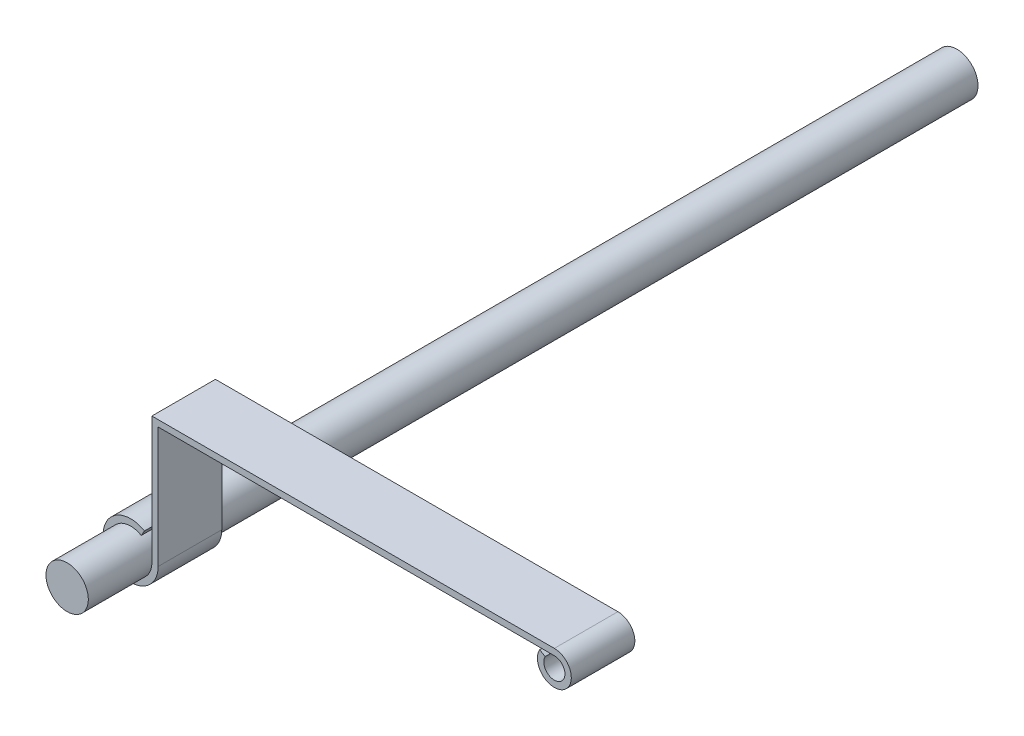
from build123d import *

# Parameters (mm, degrees)
SKETCH1_W           = 10
SKETCH1_H           = 30
BOSS_EXTRUDE1_START = 30
BOSS_EXTRUDE1_DEPTH = 30
BOSS_EXTRUDE2_START = 360
SKETCH3_R           = 10
BOSS_EXTRUDE2_DEPTH = 360


with BuildPart() as part:
    # Sketch1 → Revolve1 (revolve)
    with BuildSketch(Plane(origin=(0, 0, 0), x_dir=(1, 0, 0), z_dir=(0, 1, 0))):
        with Locations((5, -30)):
            Rectangle(SKETCH1_W, SKETCH1_H)
    revolve(axis=Axis((0, 0, 15), (0, 0, 1)))

    # Sketch2 → Boss-Extrude1 (add)
    with BuildSketch(Plane(origin=(0, 0, 15), x_dir=(-1, 0, 0), z_dir=(0, 0, -1)).offset(BOSS_EXTRUDE1_START)):
        with BuildLine():
            Line((-5, 8.660254038), (-6.5, 11.258330249))
            ThreePointArc((-6.5, 11.258330249), (11.258330249, -6.5), (-13, 0))
            Line((-13, 0), (-13, 57))
            Line((-13, 57), (-200, 57))
            ThreePointArc((-200, 57), (-202.5, 47.669872981), (-195.669872981, 54.5))
            Line((-195.669872981, 54.5), (-193.07179677, 56))
            ThreePointArc((-193.07179677, 56), (-204, 45.07179677), (-200, 60))
            Line((-200, 60), (-10, 60))
            Line((-10, 60), (-10, 0))
            ThreePointArc((-10, 0), (-8.660254038, 5), (-5, 8.660254038))
        make_face()
    extrude(amount=-BOSS_EXTRUDE1_DEPTH)

    # Sketch3 → Boss-Extrude2 (add)
    with BuildSketch(Plane(origin=(0, 0, -15), x_dir=(-1, 0, 0), z_dir=(0, 0, -1)).offset(BOSS_EXTRUDE2_START)):
        with Locations(Location((0, 0, 0), (0, 0, 180))):
            Circle(SKETCH3_R)
    extrude(amount=-BOSS_EXTRUDE2_DEPTH)


solid = part.part
